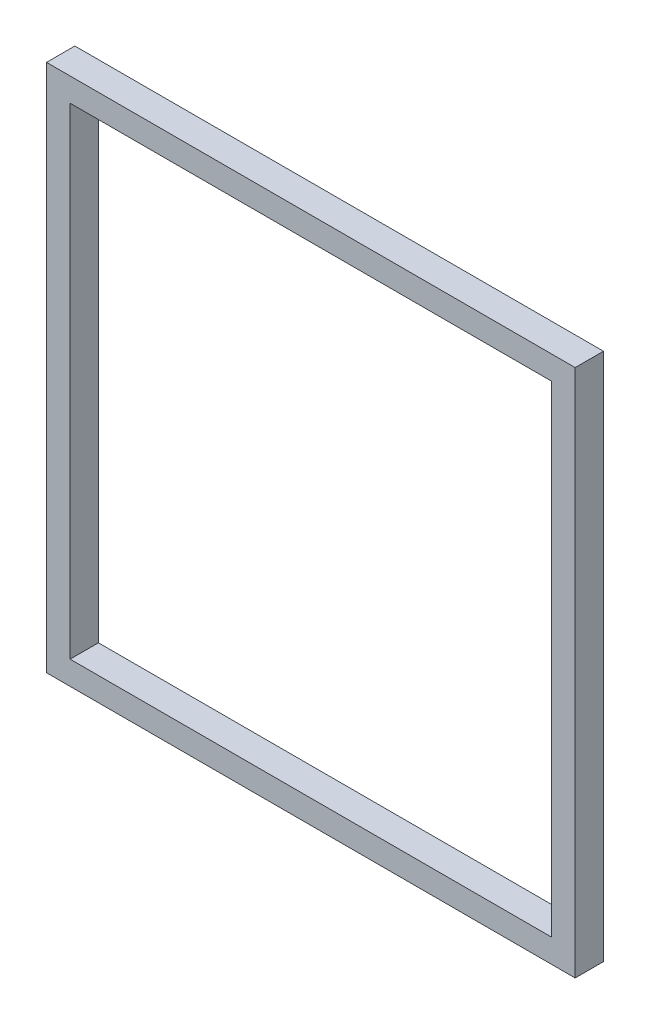
SolidWorks part; units mm, degrees
ref_plane "Front Plane" through (0, 0, 0) normal (0, 0, 1) x (1, 0, 0)
ref_plane "Top Plane" through (0, 0, 0) normal (0, 1, 0) x (1, 0, 0)
ref_plane "Right Plane" through (0, 0, 0) normal (1, 0, 0) x (0, 0, -1)
other "Configuration Table"
sketch "Sketch1" plane through (0, 0, 0) normal (0, 0, 1) x (1, 0, 0)
  line L0 (25, 535) -> (535, 535)
  line L1 (0, 0) -> (560, 0)
  line L2 (0, 0) -> (0, 560)
  line L3 (0, 560) -> (560, 560)
  line L4 (560, 0) -> (560, 560)
  line L5 (535, 25) -> (535, 535)
  line L6 (25, 25) -> (535, 25)
  line L7 (25, 25) -> (25, 535)
  dimension "D1" = 560
  dimension "D2" = 560
  dimension "D3" = 25
extrude "Boss-Extrude1" add sketch "Sketch1" along normal blind 30
